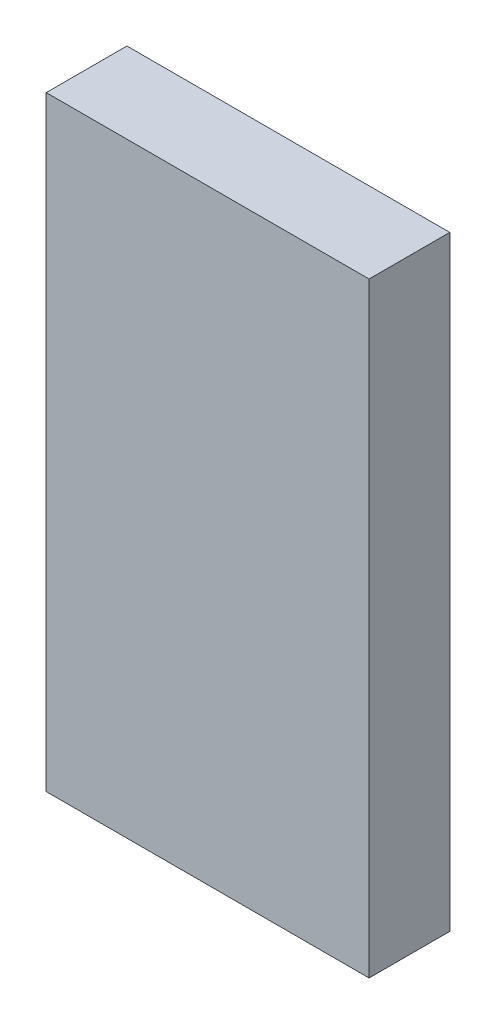
SolidWorks part; units mm, degrees
ref_plane "Front Plane" through (0, 0, 0) normal (0, 0, 1) x (1, 0, 0)
ref_plane "Top Plane" through (0, 0, 0) normal (0, 1, 0) x (1, 0, 0)
ref_plane "Right Plane" through (0, 0, 0) normal (1, 0, 0) x (0, 0, -1)
sketch "Sketch1" plane through (0, 0, 0) normal (0, 0, 1) x (1, 0, 0)
  line L1 (40, -75) -> (-40, -75)
  line L2 (40, -75) -> (40, 75)
  line L3 (40, 75) -> (-40, 75)
  line L4 (-40, -75) -> (-40, 75)
  line L5 (40, -75) -> (-40, 75) construction
  line L6 (40, 75) -> (-40, -75) construction
  point P0 (0, 0)
  dimension "D1" = 80
  dimension "D2" = 150
extrude "Boss-Extrude1" add sketch "Sketch1" along normal blind 20
